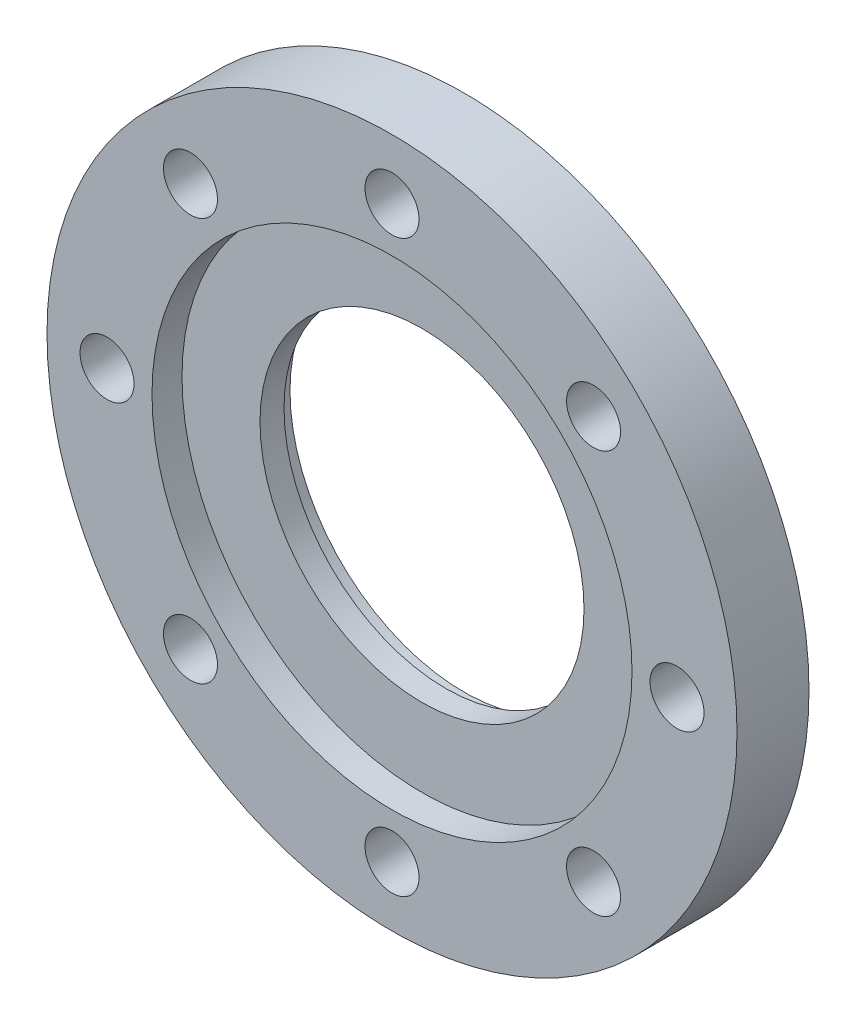
SolidWorks part; units mm, degrees
material "1023 碳钢板 (SS)"
ref_plane "前视基准面" through (0, 0, 0) normal (0, 0, 1) x (1, 0, 0)
ref_plane "上视基准面" through (0, 0, 0) normal (0, 1, 0) x (1, 0, 0)
ref_plane "右视基准面" through (0, 0, 0) normal (1, 0, 0) x (0, 0, -1)
sketch "草图1" plane through (0, 0, 0) normal (0, 0, 1) x (1, 0, 0)
  circle A0 centre (0, 0) radius 57.5
  dimension "D1" = 115
extrude "凸台-拉伸1" add sketch "草图1" along normal blind 12
sketch "草图2" plane through (0, 0, 12) normal (0, 0, 1) x (1, 0, 0)
  circle A0 centre (0, 0) radius 40
  dimension "D1" = 80
extrude "切除-拉伸1" cut sketch "草图2" against normal blind 5
sketch "草图3" plane through (0, 0, 7) normal (0, 0, 1) x (1, 0, 0)
  circle A0 centre (0, 0) radius 27
  dimension "D1" = 54
extrude "切除-拉伸2" cut sketch "草图3" against normal blind 13
sketch "草图4" plane through (0, 0, 0) normal (0, 0, -1) x (-1, 0, 0)
  circle A0 centre (0, 0) radius 29
  dimension "D1" = 58
extrude "切除-拉伸3" cut sketch "草图4" against normal blind 3
sketch "草图5" plane through (0, 0, 12) normal (0, 0, 1) x (1, 0, 0)
  circle A0 centre (0, 0) radius 47.5 construction
  circle A1 centre (0, 47.5) radius 4.5
  circle A2 centre (33.5876, 33.5876) radius 4.5
  circle A3 centre (47.5, 0) radius 4.5
  circle A4 centre (33.5876, -33.5876) radius 4.5
  circle A5 centre (0, -47.5) radius 4.5
  circle A6 centre (-33.5876, -33.5876) radius 4.5
  circle A7 centre (-47.5, 0) radius 4.5
  circle A8 centre (-33.5876, 33.5876) radius 4.5
  point P22 (0, 0)
  dimension "D1" = 95
  dimension "D2" = 9
  dimension "D3" = 8
extrude "切除-拉伸4" cut sketch "草图5" against normal blind 50
